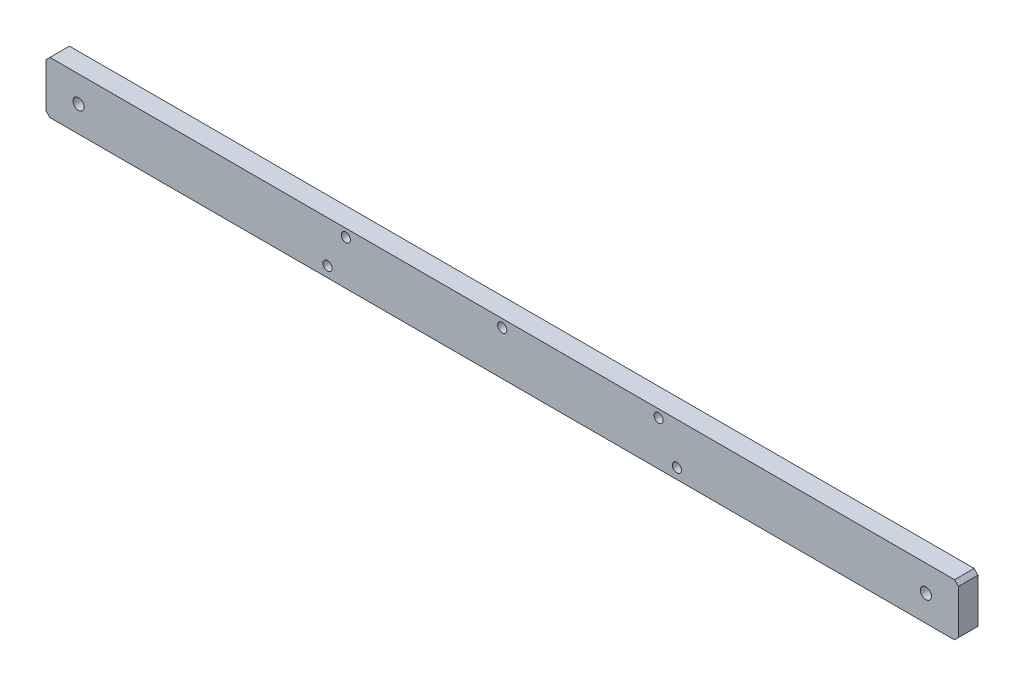
SolidWorks part; units mm, degrees
ref_plane "前视" through (0, 0, 0) normal (0, 0, 1) x (1, 0, 0)
ref_plane "上视" through (0, 0, 0) normal (0, 1, 0) x (1, 0, 0)
ref_plane "右视" through (0, 0, 0) normal (1, 0, 0) x (0, 0, -1)
sketch "草图1" plane through (0, 0, 0) normal (0, 0, 1) x (1, 0, 0)
  line L1 (0, 0) -> (700, 0)
  line L2 (0, 0) -> (0, -40)
  line L3 (0, -40) -> (700, -40)
  line L4 (700, 0) -> (700, -40)
  dimension "D1" = 700
  dimension "D2" = 40
extrude "凸台-拉伸1" add sketch "草图1" along normal blind 15
chamfer "倒角1" distance 3 angle 45 4 edges at (700, -40, 7.5) (700, 0, 7.5) (0, -40, 7.5) (0, 0, 7.5)
hole_wizard "M10 螺纹孔1" positions "草图5" profile "草图6" tap size "M10" standard "GB" end condition through all
sketch "草图5" plane through (0, 0, 15) normal (0, 0, 1) x (1, 0, 0)
  line L4 (25, -20) -> (65, -20) construction
  line L8 (0, -3) -> (0, -37) construction
  line L9 (25, -20) -> (0, -20) construction
  line L10 (700, -37) -> (700, -3) construction
  point P0 (25, -20)
  point P32 (675, -20)
  dimension "D1" = 25
  dimension "D2" = 25
sketch "草图6" plane through (25, -20, 15) normal (1, 0, 0) x (0, -1, 0)
  line L0 (0, 0) -> (0, 15)
  line L1 (0, 15) -> (4.25, 15)
  line L2 (4.25, 15) -> (4.25, 0)
  line L5 (4.25, 0) -> (0, 0)
  line L11 (0, -6.35) -> (0, 107.95) construction
  dimension "通孔螺纹孔钻头直径" = 8.5
  dimension "通孔螺纹孔钻头深度" = 15
cosmetic thread "孔螺蚊线8"
cosmetic thread "孔螺蚊线9"
hole_wizard "Ø7.0 (7) 直径孔1" positions "草图8" profile "草图7" hole size "Ø7.0" standard "ISO" end condition through all
sketch "草图8" plane through (0, 0, 15) normal (0, 0, 1) x (1, 0, 0)
  line L0 (350, 0) -> (350, -109.9698) construction
  line L1 (697, 0) -> (3, 0) construction
  point P0 (470, -6)
  point P3 (350, -6)
  point P6 (230, -6)
  point P9 (216, -32)
  point P12 (484, -32)
  dimension "D1" = 240
  dimension "D2" = 268
  dimension "D3" = 6
  dimension "D4" = 26
sketch "草图7" plane through (470, -6, 15) normal (1, 0, 0) x (0, -1, 0)
  line L0 (0, 0) -> (0, 15)
  line L1 (0, 15) -> (3.5, 15)
  line L2 (3.5, 15) -> (3.5, 0)
  line L5 (3.5, 0) -> (0, 0)
  line L11 (0, -6.35) -> (0, 107.95) construction
  dimension "通孔孔直径" = 7
  dimension "通孔孔深度" = 15
